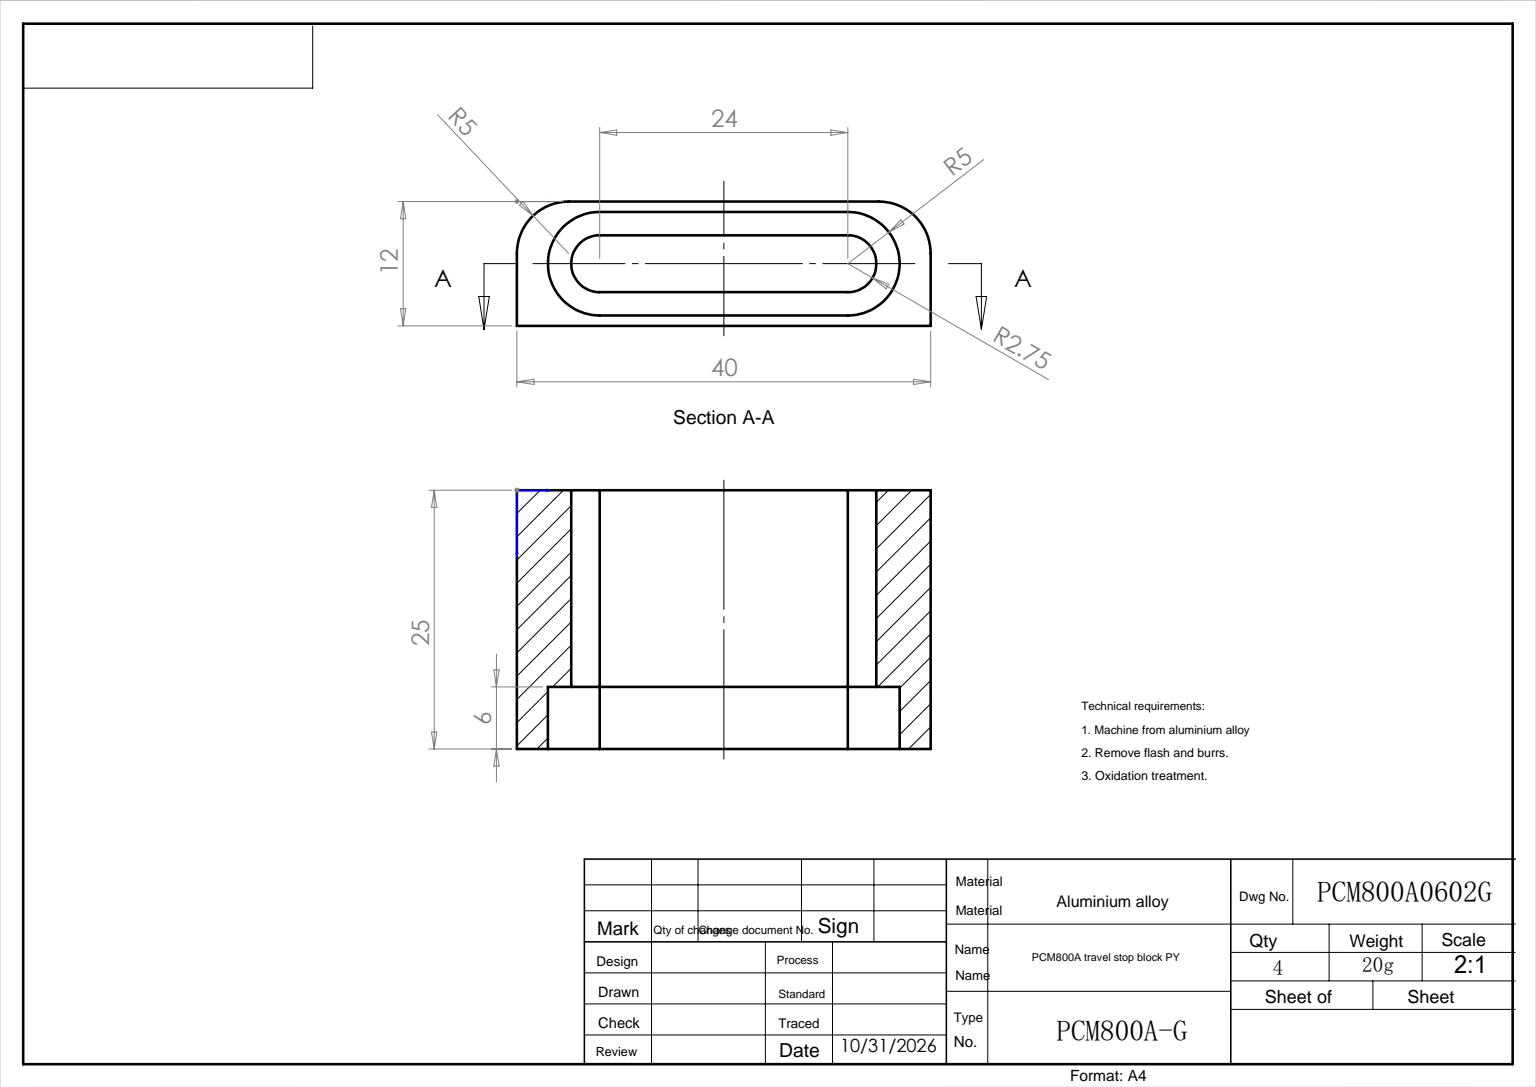
from build123d import *

# Parameters (mm, degrees)
SKETCH_1_W          = 40
SKETCH_1_H          = 25
EXTRUDE_1_DEPTH     = 12
CUT_EXTRUDE_1_DEPTH = 6
CUT_EXTRUDE_2_DEPTH = 19
FILLET_1_R          = 5


with BuildPart() as part:
    # 草图1 → 凸台-拉伸1 (new body)
    with BuildSketch(Plane.XY):
        with Locations((20, 12.5)):
            Rectangle(SKETCH_1_W, SKETCH_1_H)
    extrude(amount=EXTRUDE_1_DEPTH)

    # 草图4 → 切除-拉伸1 (cut)
    with BuildSketch(Plane(origin=(0, 25, 0), x_dir=(1, 0, 0), z_dir=(0, 1, 0))):
        with BuildLine():
            Line((8, -1), (32, -1))
            ThreePointArc((32, -1), (37, -6), (32, -11))
            Line((32, -11), (8, -11))
            ThreePointArc((8, -11), (3, -6), (8, -1))
        make_face()
    extrude(amount=-CUT_EXTRUDE_1_DEPTH, mode=Mode.SUBTRACT)

    # 草图5 → 切除-拉伸2 (cut)
    with BuildSketch(Plane(origin=(0, 19, 0), x_dir=(1, 0, 0), z_dir=(0, 1, 0))):
        with BuildLine():
            Line((8, -8.75), (32, -8.75))
            ThreePointArc((32, -8.75), (34.75, -6), (32, -3.25))
            Line((32, -3.25), (8, -3.25))
            ThreePointArc((8, -3.25), (5.25, -6), (8, -8.75))
        make_face()
    extrude(amount=-CUT_EXTRUDE_2_DEPTH, mode=Mode.SUBTRACT)

    # 圆角1
    fillet_1_edges = [part.edges().sort_by_distance(p)[0] for p in [
        (40, 12.5, 0),
        (0, 12.5, 0),
    ]]
    fillet(fillet_1_edges, radius=FILLET_1_R)


solid = part.part
